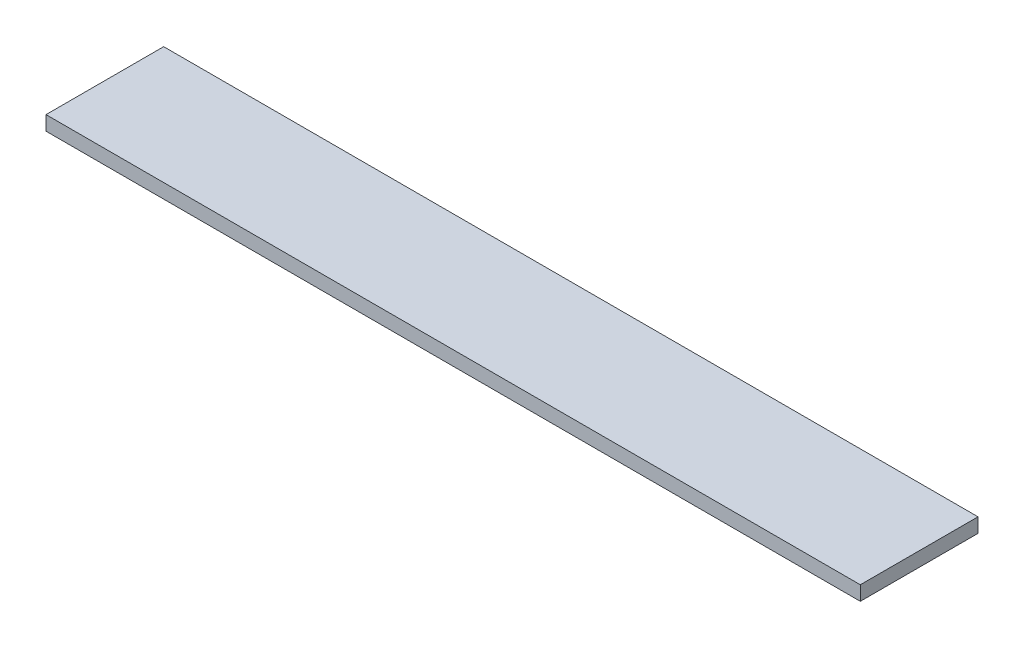
from build123d import *

# Parameters (mm, degrees)
SKETCH_1_W      = 2266
SKETCH_1_H      = 327.5
EXTRUDE_1_DEPTH = 40


with BuildPart() as part:
    # 草图1 → 凸台-拉伸1 (new body)
    with BuildSketch(Plane(origin=(0, 0, 0), x_dir=(1, 0, 0), z_dir=(0, 1, 0))):
        Rectangle(SKETCH_1_W, SKETCH_1_H)
    extrude(amount=EXTRUDE_1_DEPTH)


solid = part.part
